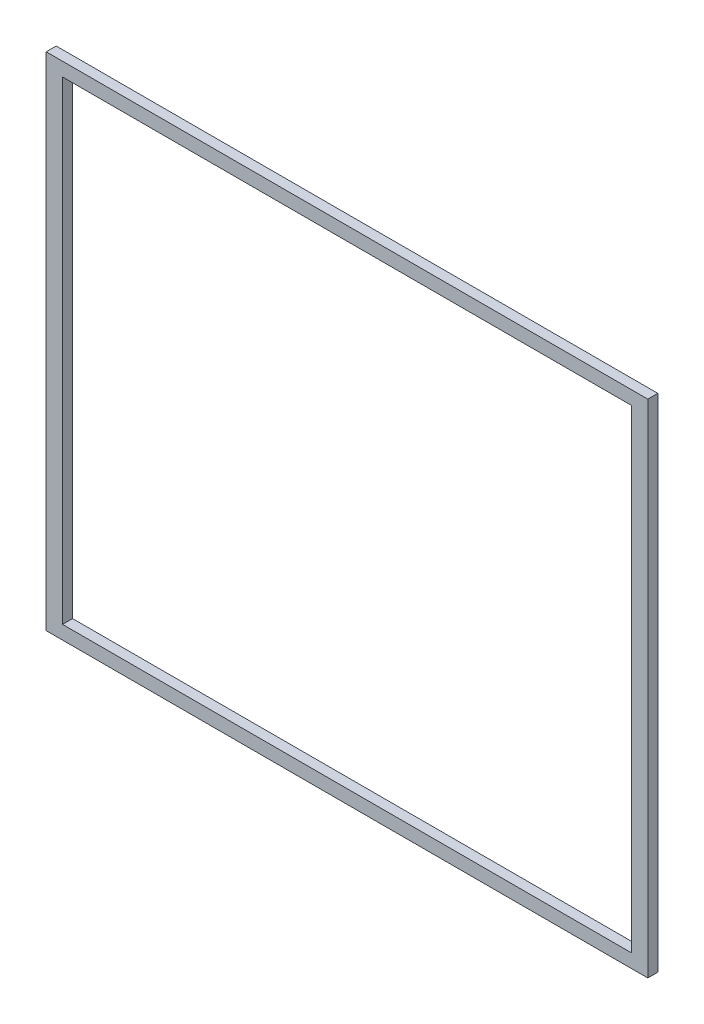
SolidWorks part; units mm, degrees
ref_plane "Front Plane" through (0, 0, 0) normal (0, 0, 1) x (1, 0, 0)
ref_plane "Top Plane" through (0, 0, 0) normal (0, 1, 0) x (1, 0, 0)
ref_plane "Right Plane" through (0, 0, 0) normal (1, 0, 0) x (0, 0, -1)
sketch "Sketch1" plane through (0, 0, 0) normal (0, 0, 1) x (1, 0, 0)
  line L1 (-300, 250) -> (300, 250)
  line L2 (-300, 250) -> (-300, -250)
  line L3 (-300, -250) -> (300, -250)
  line L4 (300, 250) -> (300, -250)
  line L5 (-300, 250) -> (300, -250) construction
  line L6 (-300, -250) -> (300, 250) construction
  line L7 (-283.6951, 236.4126) -> (283.6951, 236.4126)
  line L8 (-283.6951, 236.4126) -> (-283.6951, -236.4126)
  line L9 (-283.6951, -236.4126) -> (283.6951, -236.4126)
  line L10 (283.6951, 236.4126) -> (283.6951, -236.4126)
  line L11 (-283.6951, 236.4126) -> (283.6951, -236.4126) construction
  line L12 (-283.6951, -236.4126) -> (283.6951, 236.4126) construction
  point P0 (0, 0)
  point P6 (0, 0)
  dimension "D1" = 500
  dimension "D2" = 600
extrude "Boss-Extrude1" add sketch "Sketch1" along normal blind 10
